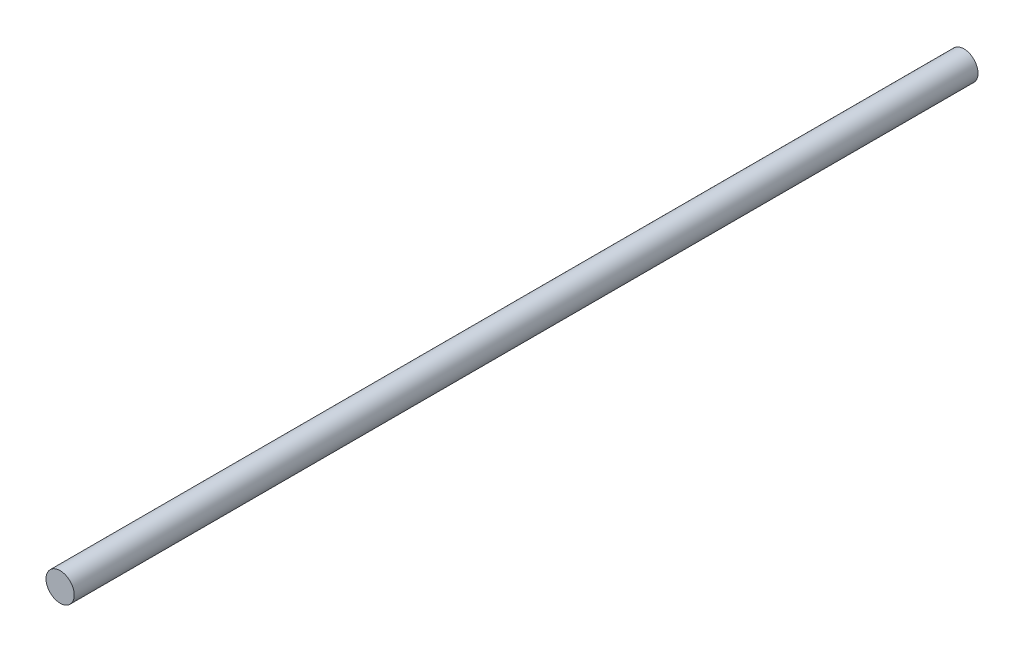
from build123d import *

# Parameters (mm, degrees)
SKETCH1_R           = 5
BOSS_EXTRUDE1_DEPTH = 320


with BuildPart() as part:
    # Sketch1 → Boss-Extrude1 (new body)
    with BuildSketch(Plane.XY):
        with Locations(Location((0, 0, 0), (0, 0, 180))):
            Circle(SKETCH1_R)
    extrude(amount=BOSS_EXTRUDE1_DEPTH)


solid = part.part
